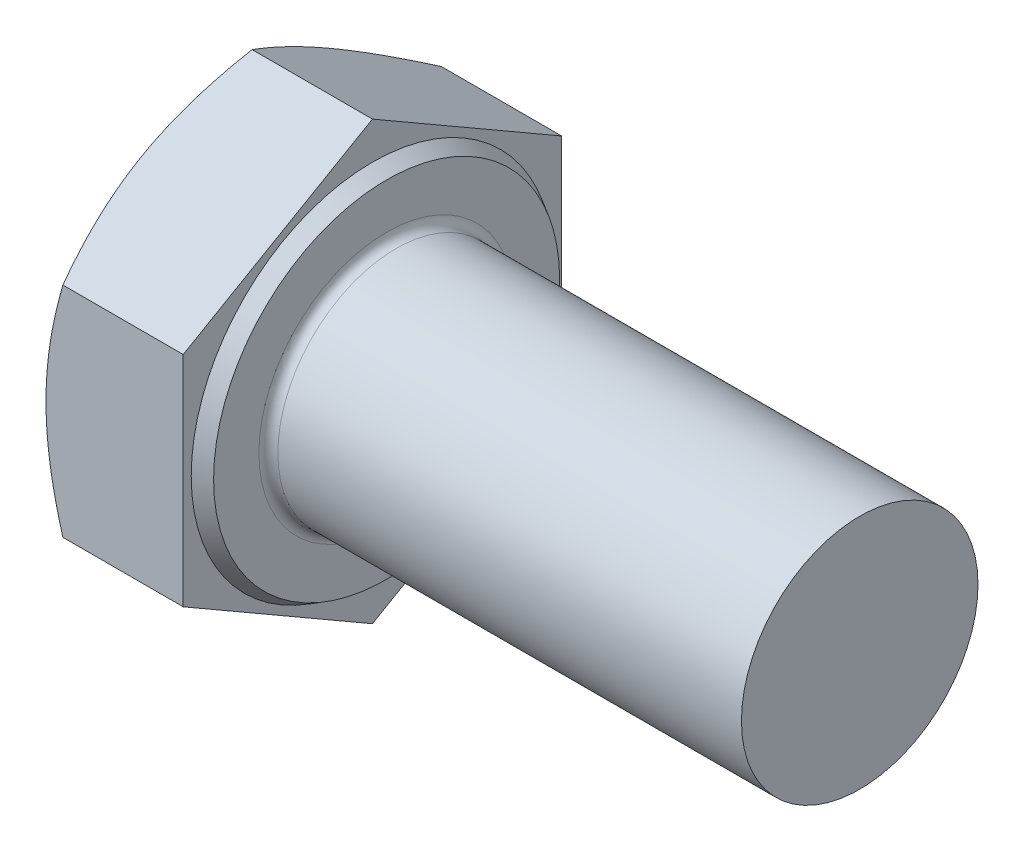
SolidWorks part; units mm, degrees
ref_plane "前视" through (0, 0, 0) normal (0, 0, 1) x (1, 0, 0)
ref_plane "上视" through (0, 0, 0) normal (0, 1, 0) x (1, 0, 0)
ref_plane "右视" through (0, 0, 0) normal (1, 0, 0) x (0, 0, -1)
sketch "草图1" plane through (0, 0, 0) normal (1, 0, 0) x (0, 0, -1)
  line L0 (8, 4.6188) -> (8, -4.6188)
  line L1 (-8, 4.6188) -> (-8, -4.6188)
  line L2 (8, -4.6188) -> (0, -9.2376)
  line L3 (0, -9.2376) -> (-8, -4.6188)
  line L4 (8, 4.6188) -> (0, 9.2376)
  line L5 (0, 9.2376) -> (-8, 4.6188)
  circle A0 centre (0, 0) radius 8.885 construction
  dimension "e" = 17.77
  dimension "s" = 16
  dimension "D2" = 120
  dimension "D3" = 8
  dimension "D4" = 8
  dimension "D5" = 8
extrude "基体-拉伸" add sketch "草图1" along normal blind 6.4
sketch "草图2" plane through (0, 0, 0) normal (0, 0, 1) x (1, 0, 0)
  line L0 (0, 4.6188) -> (0, -4.6188) construction
  line L1 (0, 0) -> (26.4, 0)
  line L2 (0, 0) -> (0, 5)
  line L3 (0, 5) -> (11.4, 5)
  line L4 (26.4, 0) -> (26.4, 3.701)
  line L5 (6.4, 9.2376) -> (6.4, 4.6188) construction
  line L7 (0, 0) -> (36.4, 0) construction
  line L8 (26.4, -3.701) -> (11.4, -5) construction
  line L9 (0, -5) -> (11.4, -5) construction
  line L10 (7.9, 5) -> (7.9, 0) construction
  line L11 (11.4, 15.24) -> (11.4, -1.27) construction
  line L12 (6.4, 4.6188) -> (6.4, -4.6188) construction
  line L13 (11.4, 5) -> (26.4, 5)
  line L14 (26.4, 5) -> (26.4, 3.701)
  dimension "l" = 20
  dimension "d" = 10
  dimension "Minor_dia" = 7.402
  dimension "p" = 1.5
  dimension "b" = 15
  dimension "ds" = 10
revolve "凸台-旋转1" add sketch "草图2" angle 360 about L7
cosmetic thread "螺旋线1" parameters "Thread_length"=26, "Thread_minor"=7.402
sketch "草图3" plane through (0, 0, 0) normal (0, 0, 1) x (1, 0, 0)
  line L0 (0, 8) -> (3.6013, 14.2376)
  line L1 (0, 9.2376) -> (0, 4.6188) construction
  line L2 (3.6013, 14.2376) -> (3.6013, 19.2376)
  line L3 (3.6013, 19.2376) -> (-10, 19.2376)
  line L4 (-10, 19.2376) -> (-10, 8)
  line L5 (-10, 8) -> (0, 8)
  line L6 (0, 0) -> (99.06, 0) construction
  line L7 (6.4, 9.2376) -> (0, 9.2376) construction
  dimension "D1" = 8
  dimension "D2" = 5
  dimension "D3" = 10
  dimension "D4" = 5
  dimension "Head_ch_ang" = 30
revolve "切除-旋转1" cut sketch "草图3" angle 360 about L6
sketch "草图4" plane through (0, 0, 0) normal (0, 0, 1) x (1, 0, 0)
  line L0 (6.4, 0) -> (6.4, 7.315) construction
  line L2 (6.4, -5) -> (6.4, 5) construction
  line L3 (6.4, 9.2376) -> (6.4, 4.6188) construction
  line L4 (6.4, 7.315) -> (5.8, 7.6614)
  line L5 (0, 0) -> (95.25, 0) construction
  line L6 (0, 0) -> (36.4, 0) construction
  line L9 (5.8, 7.6614) -> (5.8, 9.2376)
  line L10 (6.4, 9.2376) -> (0.7145, 9.2376) construction
  line L11 (5.8, 9.2376) -> (6.4, 9.2376)
  line L12 (6.4, 9.2376) -> (6.4, 7.315)
  dimension "D1" = 120
  dimension "c" = 0.6
  dimension "dw" = 14.63
revolve "切除-旋转3" cut sketch "草图4" angle 360 about L5
fillet "圆角" radius 0.4 1 edges at (6.4, 0, -5)
sketch "草图6" plane through (0, 0, 0) normal (0, 0, 1) x (1, 0, 0)
  line L0 (0, 0) -> (26.4, 0) construction
  line L1 (26.4, -5) -> (26.4, 5) construction
  line L2 (26.4, 0) -> (26.4, 5) construction
  line L4 (25.65, 5) -> (27.15, 5)
  line L5 (25.65, 5) -> (26.4, 3.701)
  line L6 (26.4, 3.701) -> (27.15, 5)
  dimension "D1" = 1.5
revolve "切除-旋转4" [suppressed] cut sketch "草图6" angle 360 about L0
pattern_linear "阵列(线性)1" [suppressed]
